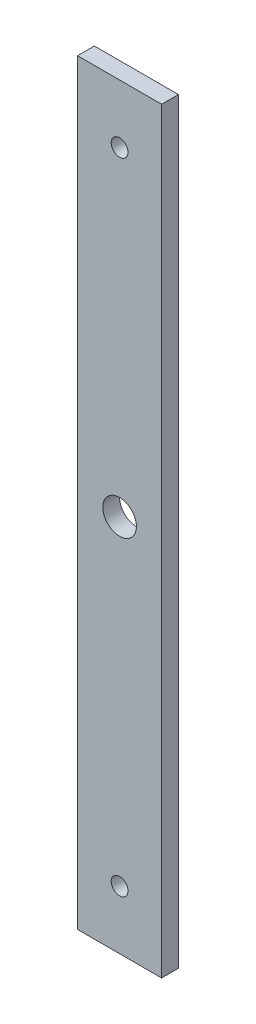
SolidWorks part; units mm, degrees
ref_plane "前视基准面" through (0, 0, 0) normal (0, 0, 1) x (1, 0, 0)
ref_plane "上视基准面" through (0, 0, 0) normal (0, 1, 0) x (1, 0, 0)
ref_plane "右视基准面" through (0, 0, 0) normal (1, 0, 0) x (0, 0, -1)
other "Configuration Table"
sketch "草图1" plane through (0, 0, 0) normal (0, 0, 1) x (1, 0, 0)
  line L0 (0, 0) -> (0, 450)
  line L1 (0, 450) -> (50, 450)
  line L2 (50, 450) -> (50, 0)
  line L3 (50, 0) -> (0, 0)
  line L4 (50, 225) -> (0, 225) construction
  line L5 (25, 450) -> (25, 0) construction
  circle A0 centre (25, 225) radius 10
  circle A1 centre (25, 415.2012) radius 5
  circle A2 centre (25, 34.7988) radius 5
  dimension "D3" = 20
  dimension "D1" = 50
  dimension "D2" = 450
extrude "凸台-拉伸1" add sketch "草图1" along normal blind 10
